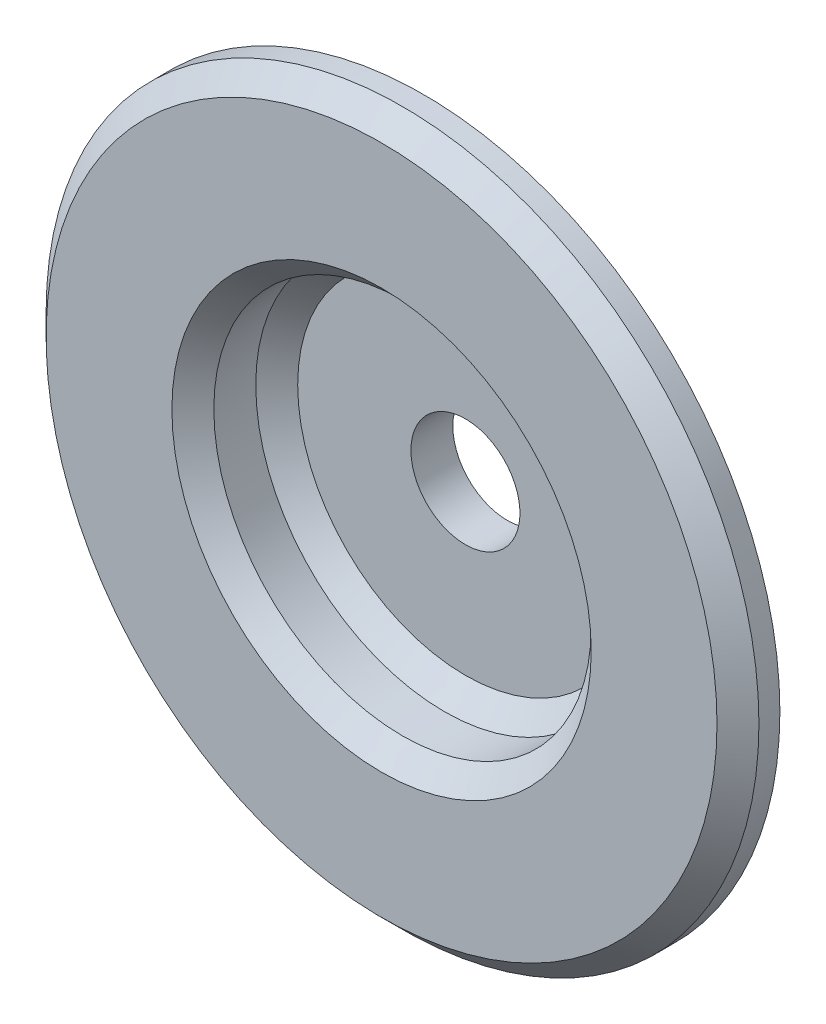
from build123d import *

# Parameters (mm, degrees)
SKETCH_1_R      = 11
SKETCH_1_R_2    = 9
EXTRUDE_1_DEPTH = 6
SKETCH_2_R      = 11
SKETCH_2_R_2    = 2.6
EXTRUDE_2_DEPTH = 2
CHAMFER_1_SIZE  = 1
EXTRUDE_START   = -2
SKETCH_3_R      = 17
SKETCH_3_R_2    = 9
EXTRUDE_3_DEPTH = 2
CHAMFER_2_SIZE  = 1


with BuildPart() as part:
    # 草图1 → 凸台-拉伸1 (new body)
    with BuildSketch(Plane.XY):
        Circle(SKETCH_1_R)
        Circle(SKETCH_1_R_2, mode=Mode.SUBTRACT)
    extrude(amount=EXTRUDE_1_DEPTH)

    # 草图2 → 凸台-拉伸2 (add)
    with BuildSketch(Plane(origin=(0, 0, 0), x_dir=(-1, 0, 0), z_dir=(0, 0, -1))):
        with Locations(Location((0, 0, 0), (0, 0, 180))):
            Circle(SKETCH_2_R)
        Circle(SKETCH_2_R_2, mode=Mode.SUBTRACT)
    extrude(amount=-EXTRUDE_2_DEPTH)

    # 倒角1
    chamfer_1_edges = [part.edges().sort_by_distance(p)[0] for p in [
        (-9, 0, 2),
        (-11, 0, 0),
    ]]
    chamfer(chamfer_1_edges, length=CHAMFER_1_SIZE)

    # 草图3 → 凸台-拉伸3 (add)
    with BuildSketch(Plane.XY.offset(6).offset(EXTRUDE_START)):
        Circle(SKETCH_3_R)
        with Locations(Location((0, 0, 0), (0, 0, 180))):
            Circle(SKETCH_3_R_2, mode=Mode.SUBTRACT)
    extrude(amount=EXTRUDE_3_DEPTH)

    # 倒角2
    chamfer_2_edges = [part.edges().sort_by_distance(p)[0] for p in [
        (-17, 0, 6),
        (-9, 0, 6),
    ]]
    chamfer(chamfer_2_edges, length=CHAMFER_2_SIZE)


solid = part.part
